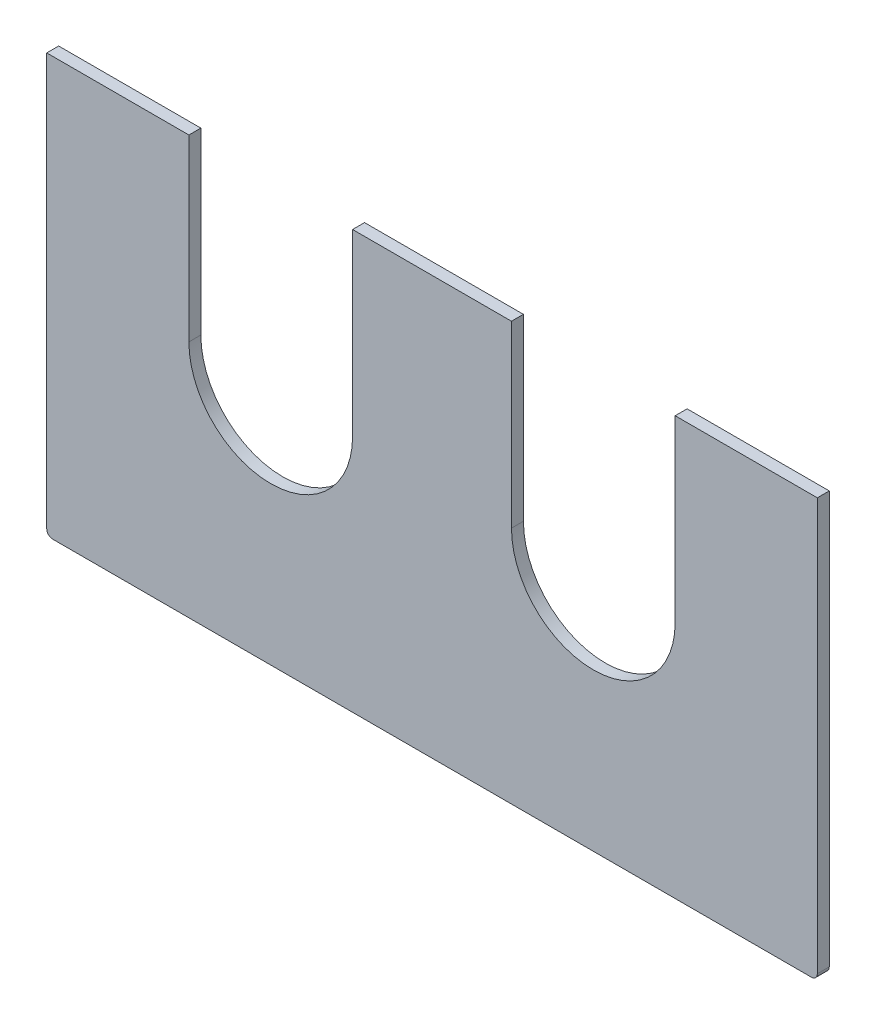
from build123d import *

# Parameters (mm, degrees)
SKETCH1_W           = 1290
SKETCH1_H           = 700
BOSS_EXTRUDE1_DEPTH = 20
CUT_EXTRUDE1_DEPTH  = 20
FILLET1_R           = 10


with BuildPart() as part:
    # Sketch1 → Boss-Extrude1 (new body)
    with BuildSketch(Plane.XY):
        Rectangle(SKETCH1_W, SKETCH1_H)
    extrude(amount=BOSS_EXTRUDE1_DEPTH)

    # Sketch2 → Cut-Extrude1 (cut)
    with BuildSketch(Plane.XY.offset(20)):
        with BuildLine():
            Line((-407, 50), (-407, 350))
            Line((-407, 350), (-133, 350))
            Line((-133, 350), (-133, 50))
            ThreePointArc((-133, 50), (-270, -87), (-407, 50))
        make_face()
        with BuildLine():
            Line((407, 350), (133, 350))
            Line((133, 350), (133, 50))
            ThreePointArc((133, 50), (270, -87), (407, 50))
            Line((407, 50), (407, 350))
        make_face()
    extrude(amount=-CUT_EXTRUDE1_DEPTH, mode=Mode.SUBTRACT)

    # Fillet1
    fillet1_edges = [part.edges().sort_by_distance(p)[0] for p in [
        (645, -350, 10),
        (-645, -350, 10),
    ]]
    fillet(fillet1_edges, radius=FILLET1_R)


solid = part.part
